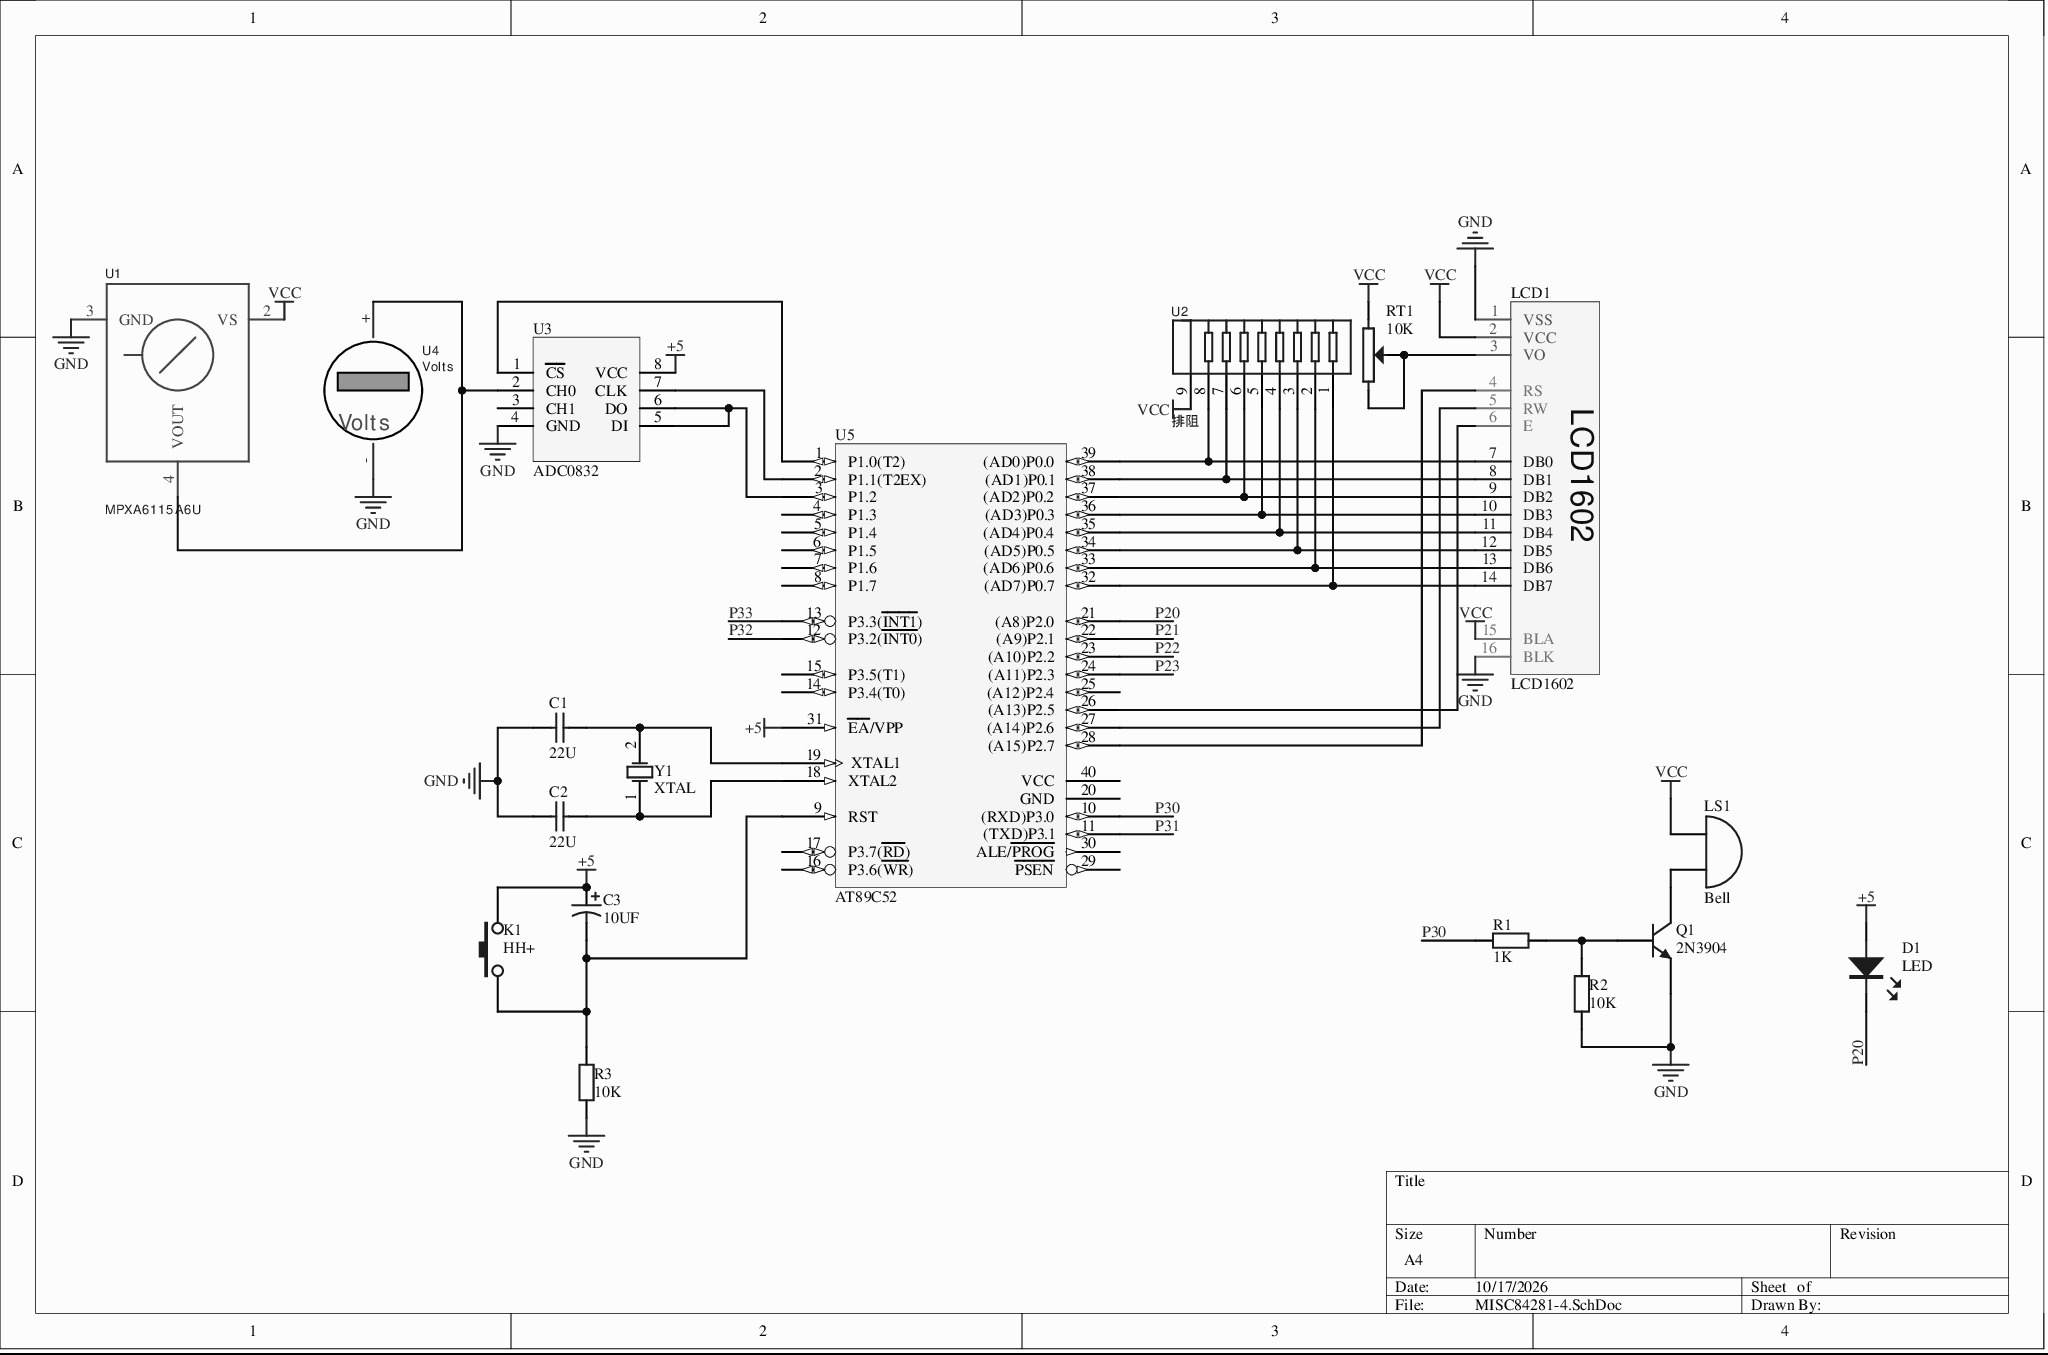
[diagram p0: MISC84281-4.SchDoc]
# Altium project MISC84281-7.PrjPcb
1 sheet, 18 parts. Net scope: global (net labels, ports and power ports of the same name join across sheets).
Board file: MISC84281.PcbDoc

## Sheet MISC84281-4.SchDoc
size A4

### Parts
C1  22U  [RAD-0.3]
C2  22U  [RAD-0.3]
C3  10UF  [RB7.6-15]
D1  LED  [LED5-BLUE]
K1  HH+  [四脚轻触开关]
LCD1  LCD1602  [LCD1602]
LS1  Bell  [PIN2]
Q1  2N3904  [TO-92A]
R1  1K  [AXIAL-0.4]
R2  10K  [AXIAL-0.4]
R3  10K  [AXIAL-0.4]
RT1  10K  [电位器]
U1  MPXA6115A6U  [482]
U2  排阻  [paizu]
U3  ADC0832  [P008]
U4  Volts  [CAPACITANCE 1 FARAD 5,5 VOLT]
U5  AT89C52  [DIP40]
Y1  XTAL  [R38]

### Nets
+5: C3.1 D1.A K1.2 U3.8(VCC) U5.31(~{EA}/VPP)
GND: C1.1 C2.1 LCD1.1(VSS) LCD1.16(BLK) Q1.1(E) R2.1 R3.1 U1.3(GND) U3.4(GND) U4.-
VCC: LCD1.2(VCC) LCD1.15(BLA) LS1.1(A) RT1.1 U1.2(VS) U2.9
P20: D1.K U5.21((A8)P2.0)
P21: U5.22((A9)P2.1)
P22: U5.23((A10)P2.2)
P23: U5.24((A11)P2.3)
P30: R1.2 U5.10((RXD)P3.0)
P31: U5.11((TXD)P3.1)
P32: U5.12(P3.2(~{INT0}))
P33: U5.13(P3.3(~{INT1}))
NetC1_2: C1.2 U5.19(XTAL1) Y1.2(OSC2)
NetC2_2: C2.2 U5.18(XTAL2) Y1.1(OSC1)
NetC3_2: C3.2 K1.1 R3.2 U5.9(RST)
NetLCD1_3: LCD1.3(VO) RT1.2 RT1.3(W)
NetLCD1_4: LCD1.4(RS) U5.28((A15)P2.7)
NetLCD1_5: LCD1.5(RW) U5.27((A14)P2.6)
NetLCD1_6: LCD1.6(E) U5.26((A13)P2.5)
NetLCD1_7: LCD1.7(DB0) U2.8 U5.39((AD0)P0.0)
NetLCD1_8: LCD1.8(DB1) U2.7 U5.38((AD1)P0.1)
NetLCD1_9: LCD1.9(DB2) U2.6 U5.37((AD2)P0.2)
NetLCD1_10: LCD1.10(DB3) U2.5 U5.36((AD3)P0.3)
NetLCD1_11: LCD1.11(DB4) U2.4 U5.35((AD4)P0.4)
NetLCD1_12: LCD1.12(DB5) U2.3 U5.34((AD5)P0.5)
NetLCD1_13: LCD1.13(DB6) U2.2 U5.33((AD6)P0.6)
NetLCD1_14: LCD1.14(DB7) U2.1 U5.32((AD7)P0.7)
NetLS1_2: LS1.2(B) Q1.3(C)
NetQ1_2: Q1.2(B) R1.1 R2.2
NetU1_4: U1.4(VOUT) U3.2(CH0) U4.+
NetU3_1: U3.1(~{CS}) U5.1(P1.0(T2))
NetU3_5: U3.5(DI) U3.6(DO) U5.3(P1.2)
NetU3_7: U3.7(CLK) U5.2(P1.1(T2EX))

Not connected (* = marked no-connect by the designer): U1 1(NC) 5(NC) 6(NC); U3 3(CH1); U5 4(P1.3) 5(P1.4) 6(P1.5) 7(P1.6) 8(P1.7) 14(P3.4(T0)) 15(P3.5(T1)) 16(P3.6(~{WR})) 17(P3.7(~{RD})) 20(GND) 25((A12)P2.4) 29(~{PSEN}) 30(ALE/~{PROG}) 40(VCC)

### Library data of the parts
C1 C2 = Cap: Capacitor; Value: 100pF; Published: 8-Jun-2000; LatestRevisionDate: 17-Jul-2002; LatestRevisionNote: Re-released for DXP Platform.; PackageReference: RAD-0.3; PackageDescription: Radial Cap, Thru-Hole; 2 Leads; 0.3 in Pin Spacing; Publisher: Altium Limited
C3 = Cap Pol1: Polarized Capacitor (Radial); Value: 100pF; Published: 8-Jun-2000; LatestRevisionDate: 17-Jul-2002; LatestRevisionNote: Re-released for DXP Platform.; PackageReference: RB7.6-15; PackageDescription: Polarized Capacitor (Radial); 2 Leads; Publisher: Altium Limited
K1 = 四脚轻触开关
LS1 = Bell: Electrical Bell; Published: 24-Mar-1999; LatestRevisionDate: 17-Jul-2002; LatestRevisionNote: Re-released for DXP Platform.; PackageReference: PIN2; Publisher: Altium Limited
Q1 = 2N3904: NPN General Purpose Amplifier; Published: 8-Jun-2000; LatestRevisionDate: 15-Jan-2003; LatestRevisionNote: PCB Footprint 'BCY-W3/D4.7' replaced; DatasheetVersion: 1997; PackageVersion: Sep-1998; PackageReference: TO-92A; PackageDescription: TO, Flat Index; 3 In-Line, Axial Leads; Body Dia. 4.5mm; Leads 0.51 x 0.48 mm (max); ComponentLink1Description: Manufacturer Link; ComponentLink2Description: Datasheet; ComponentLink2URL: http://www.fairchildsemi.com/ds/2N%2F2N3904.pdf; Publisher: Altium Limited
R1 = Res2: Resistor; Published: 8-Jun-2000; LatestRevisionDate: 17-Jul-2002; LatestRevisionNote: Re-released for DXP Platform.; PackageReference: AXIAL-0.4; PackageDescription: Axial Device, Thru-Hole; 2 Leads; 0.4 in Pin Spacing; Value: 1K; Publisher: Altium Limited
R2 R3 = Res2: Resistor; Value: 1K; Published: 8-Jun-2000; LatestRevisionDate: 17-Jul-2002; LatestRevisionNote: Re-released for DXP Platform.; PackageReference: AXIAL-0.4; PackageDescription: Axial Device, Thru-Hole; 2 Leads; 0.4 in Pin Spacing; Publisher: Altium Limited
RT1 = 电位器
U3 = ADC0832: U?
U5 = STC89C52
Y1 = XTAL: Crystal Oscillator; Published: 8-Jun-2000; LatestRevisionDate: 17-Jul-2002; LatestRevisionNote: Re-released for DXP Platform.; PackageReference: R38; PackageDescription: Crystal, Thru-Hole; 2 Leads; Body 3.1 x 8.2 mm (Dia.xH); Publisher: Altium Limited